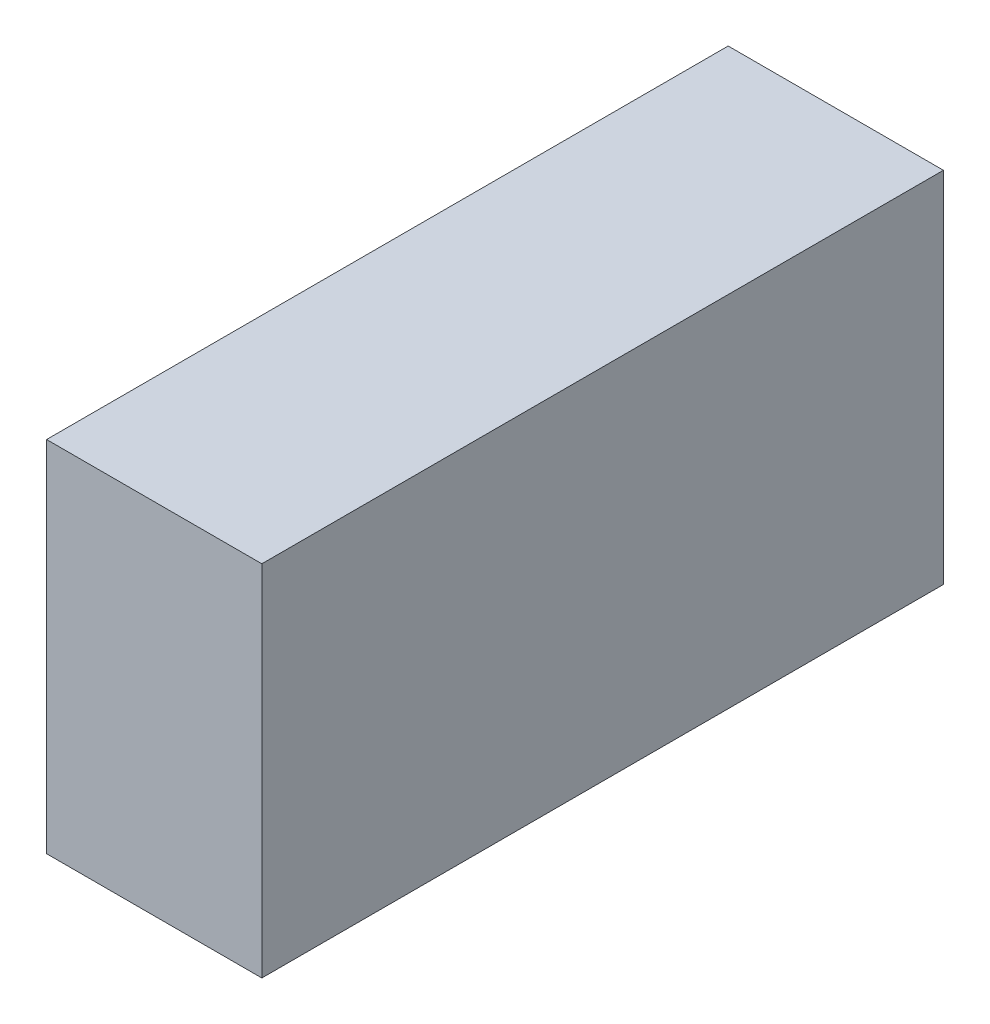
from build123d import *

# Parameters (mm, degrees)
SKETCH1_W           = 38
SKETCH1_H           = 20
BOSS_EXTRUDE1_DEPTH = 12


with BuildPart() as part:
    # Sketch1 → Boss-Extrude1 (new body)
    with BuildSketch(Plane(origin=(0, 0, 0), x_dir=(0, 0, -1), z_dir=(1, 0, 0))):
        with Locations((19, 10)):
            Rectangle(SKETCH1_W, SKETCH1_H)
    extrude(amount=BOSS_EXTRUDE1_DEPTH)


solid = part.part
